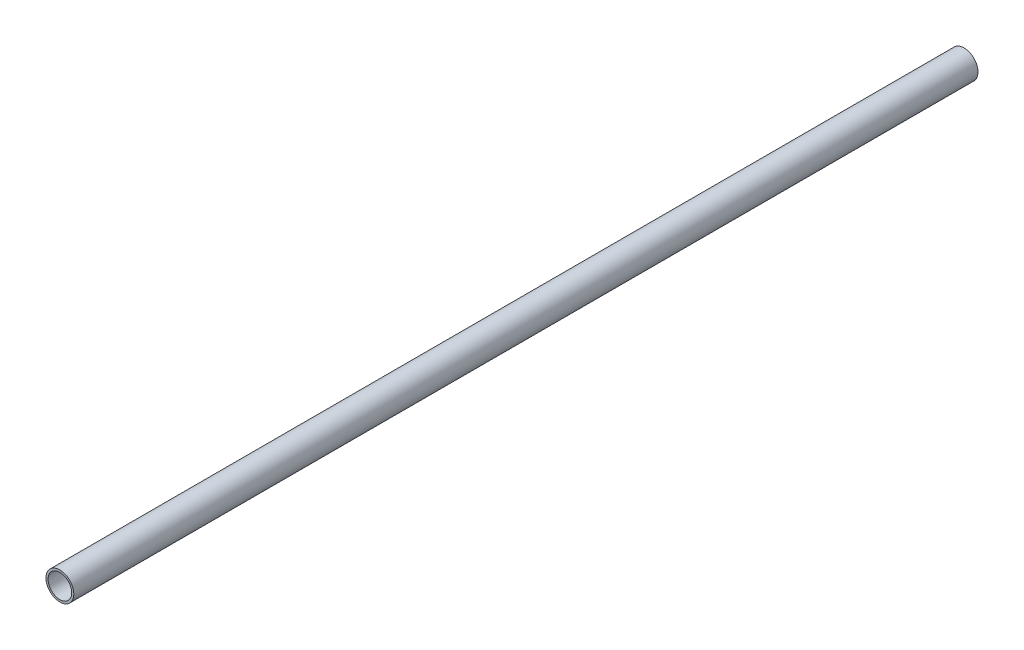
SolidWorks part; units mm, degrees
ref_plane "Front Plane" through (0, 0, 0) normal (0, 0, 1) x (1, 0, 0)
ref_plane "Top Plane" through (0, 0, 0) normal (0, 1, 0) x (1, 0, 0)
ref_plane "Right Plane" through (0, 0, 0) normal (1, 0, 0) x (0, 0, -1)
sketch "Sketch1" plane through (0, 0, 0) normal (0, 0, 1) x (1, 0, 0)
  line L1 (-12, -12) -> (12, -12) construction
  line L2 (-12, -12) -> (-12, 12) construction
  line L3 (-12, 12) -> (12, 12) construction
  line L4 (12, -12) -> (12, 12) construction
  line L5 (-12, -12) -> (12, 12) construction
  line L6 (-12, 12) -> (12, -12) construction
  circle A0 centre (0, 0) radius 20
  circle A1 centre (0, 0) radius 17
  dimension "D1" = 40
  dimension "D2" = 3
  dimension "D3" = 24
extrude "Boss-Extrude1" add sketch "Sketch1" along normal mid plane 1300
